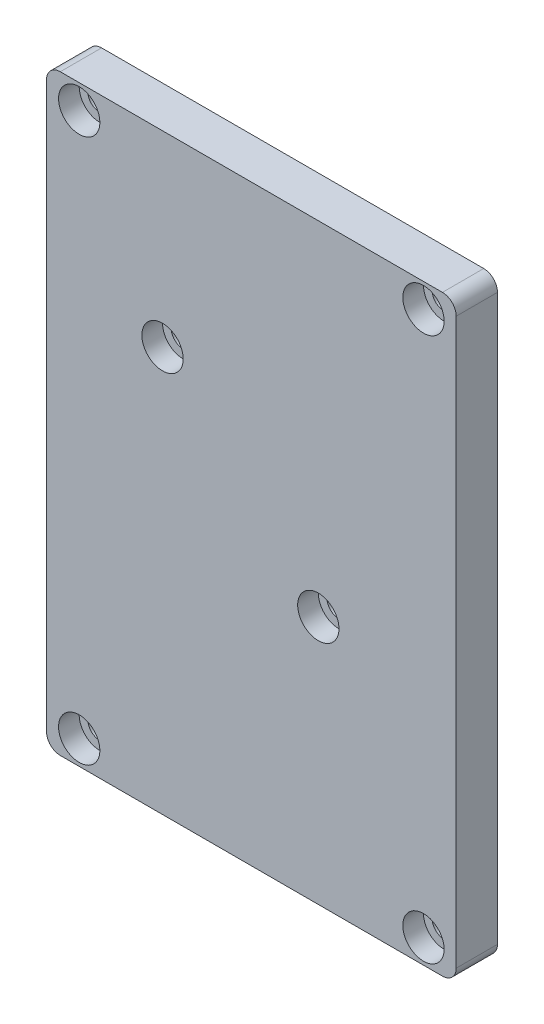
from build123d import *

# Parameters (mm, degrees)
SKETCH_1_W          = 59.5
SKETCH_1_H          = 86
EXTRUDE_1_DEPTH     = 6
SKETCH_2_R          = 1.75
CUT_EXTRUDE_1_DEPTH = 6
SKETCH_3_R          = 3
CUT_EXTRUDE_2_DEPTH = 3
FILLET_1_R          = 2


with BuildPart() as part:
    # 草图1 → 凸台-拉伸1 (new body)
    with BuildSketch(Plane.XY):
        Rectangle(SKETCH_1_W, SKETCH_1_H)
    extrude(amount=EXTRUDE_1_DEPTH)

    # 草图2 → 切除-拉伸1 (cut)
    with BuildSketch(Plane.XY.offset(6)):
        with Locations((-25, -39.5)):
            Circle(SKETCH_2_R)
        with Locations((25, -39.5)):
            Circle(SKETCH_2_R)
        with Locations((25, 39.5)):
            Circle(SKETCH_2_R)
        with Locations((-25, 39.5)):
            Circle(SKETCH_2_R)
        with Locations((-12.9, 15.8)):
            Circle(SKETCH_2_R)
        with Locations((9.727416998, -6.827416998)):
            Circle(SKETCH_2_R)
    extrude(amount=-CUT_EXTRUDE_1_DEPTH, mode=Mode.SUBTRACT)

    # 草图3 → 切除-拉伸2 (cut)
    with BuildSketch(Plane.XY.offset(6)):
        with Locations((-25, 39.5)):
            Circle(SKETCH_3_R)
        with Locations((25, 39.5)):
            Circle(SKETCH_3_R)
        with Locations((-12.9, 15.8)):
            Circle(SKETCH_3_R)
        with Locations((9.727416998, -6.827416998)):
            Circle(SKETCH_3_R)
        with Locations((-25, -39.5)):
            Circle(SKETCH_3_R)
        with Locations((25, -39.5)):
            Circle(SKETCH_3_R)
    extrude(amount=-CUT_EXTRUDE_2_DEPTH, mode=Mode.SUBTRACT)

    # 圆角1
    fillet_1_edges = [part.edges().sort_by_distance(p)[0] for p in [
        (29.75, -43, 3),
        (-29.75, -43, 3),
        (-29.75, 43, 3),
        (29.75, 43, 3),
    ]]
    fillet(fillet_1_edges, radius=FILLET_1_R)


solid = part.part
